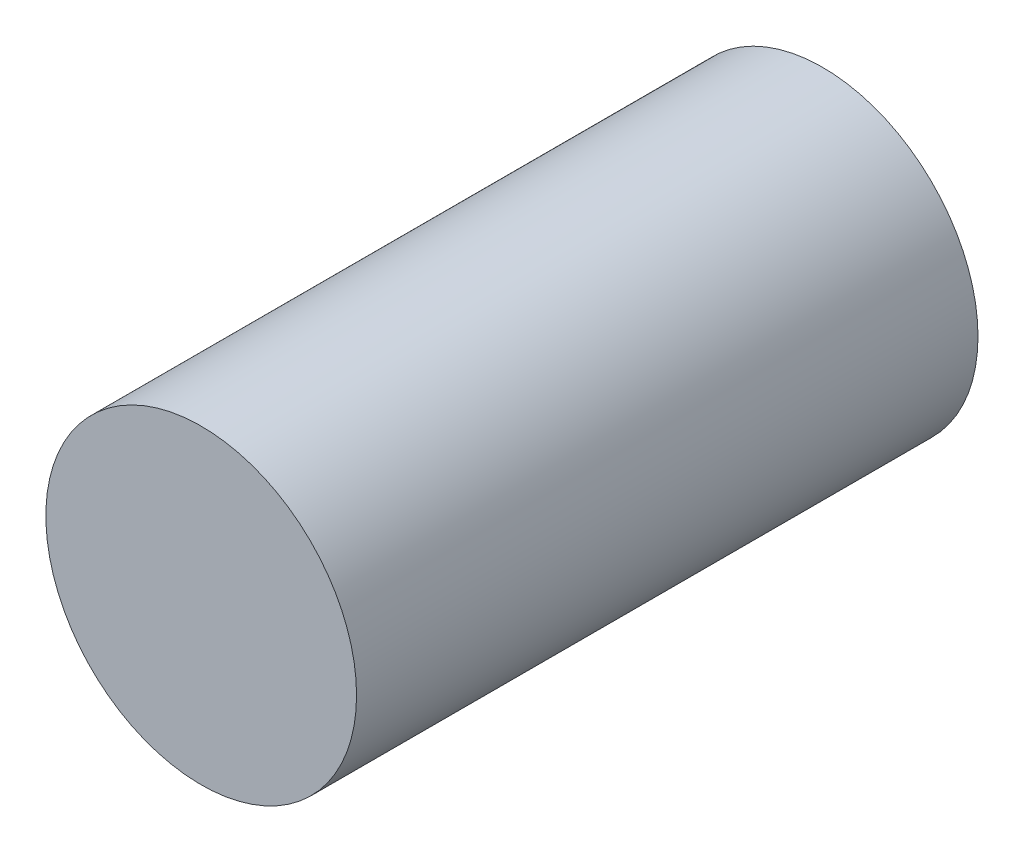
from build123d import *

# Parameters (mm, degrees)
SKETCH1_R           = 10
BOSS_EXTRUDE1_DEPTH = 20


with BuildPart() as part:
    # Sketch1 → Boss-Extrude1 (new, symmetric)
    with BuildSketch(Plane.XY):
        Circle(SKETCH1_R)
    extrude(amount=BOSS_EXTRUDE1_DEPTH, both=True)


solid = part.part
